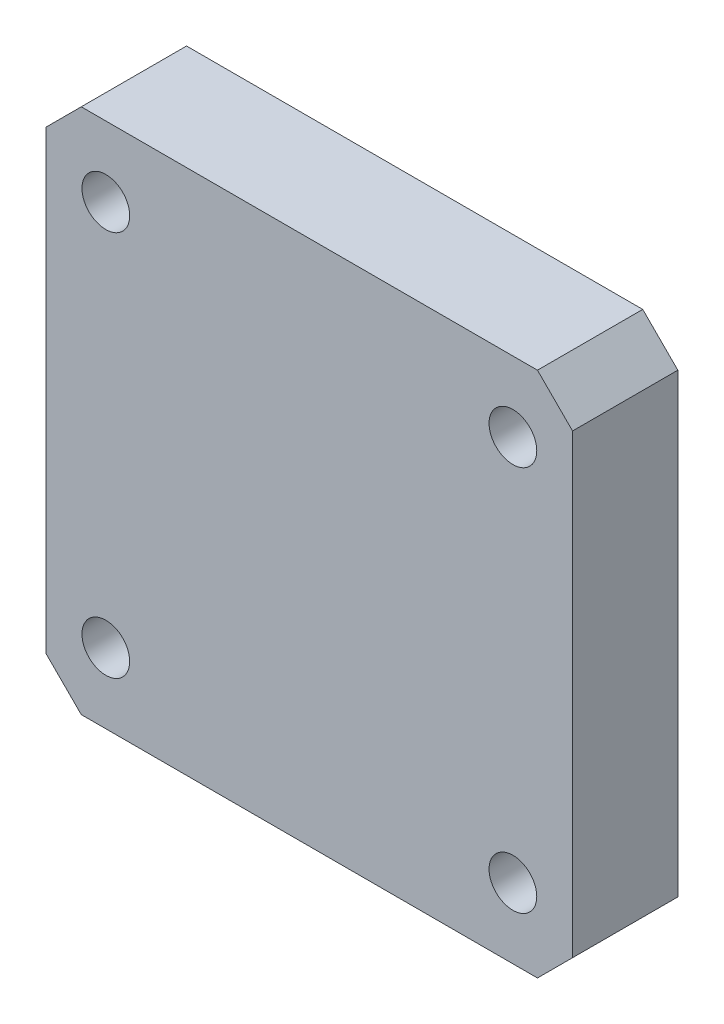
from build123d import *

# Parameters (mm, degrees)
BOSS_EXTRUDE1_DEPTH   = 15
M8_TAPPED_HOLE1_D     = 6.8
M8_TAPPED_HOLE1_DEPTH = 19.75
M8_TAPPED_HOLE1_TIP   = 2.042926105


with BuildPart() as part:
    # Sketch1 → Boss-Extrude1 (new body)
    with BuildSketch(Plane.XY):
        Polygon((-37.5, 32.5), (-32.5, 37.5), (32.5, 37.5), (37.5, 32.5), (37.5, -32.5), (32.5, -37.5), (-32.5, -37.5), (-37.5, -32.5), align=None)
    extrude(amount=BOSS_EXTRUDE1_DEPTH)

    # M8 Tapped Hole1
    with Locations(Plane.XY.offset(15)):
        with Locations((-29, 27.5), (29, 27.5), (29, -27.5), (-29, -27.5)):
            Hole(M8_TAPPED_HOLE1_D / 2, depth=M8_TAPPED_HOLE1_DEPTH)
            with Locations((0, 0, -(M8_TAPPED_HOLE1_DEPTH + M8_TAPPED_HOLE1_TIP / 2))):  # 118° drill point
                Cone(0, M8_TAPPED_HOLE1_D / 2, M8_TAPPED_HOLE1_TIP, mode=Mode.SUBTRACT)


solid = part.part
